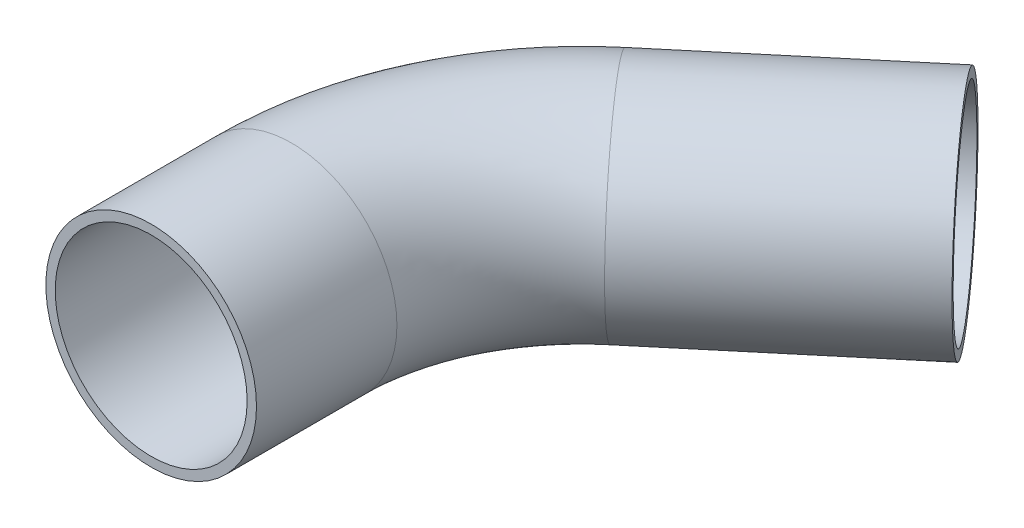
from build123d import *

# Parameters (mm, degrees)
SKETCH1_R = 22.5
SHELL1_T  = -2


with BuildPart() as part:
    # Sweep1: sweep along a path in Sketch2
    with BuildLine(Plane(origin=(0, 0, 0), x_dir=(1, 0, 0), z_dir=(0, 1, 0))) as sweep1_path:
        Line((0, 0), (0, 29.998925194))
        ThreePointArc((0, 29.998925194), (5.808917204, 56.201257422), (22.147168199, 77.493680668))
        Line((22.147168199, 77.493680668), (62.502026728, 111.355427576))
    # Sketch1 → Sweep1 (sweep)
    with BuildSketch(Plane.XY):
        Circle(SKETCH1_R)
    sweep(path=sweep1_path.line)

    # Shell1
    shell1_openings = [part.faces().sort_by_distance(p)[0] for p in [
        (62.502026728, 0, -111.355427576),
        (0, 0, 0),
    ]]
    offset(amount=SHELL1_T, openings=shell1_openings, kind=Kind.INTERSECTION)


solid = part.part
